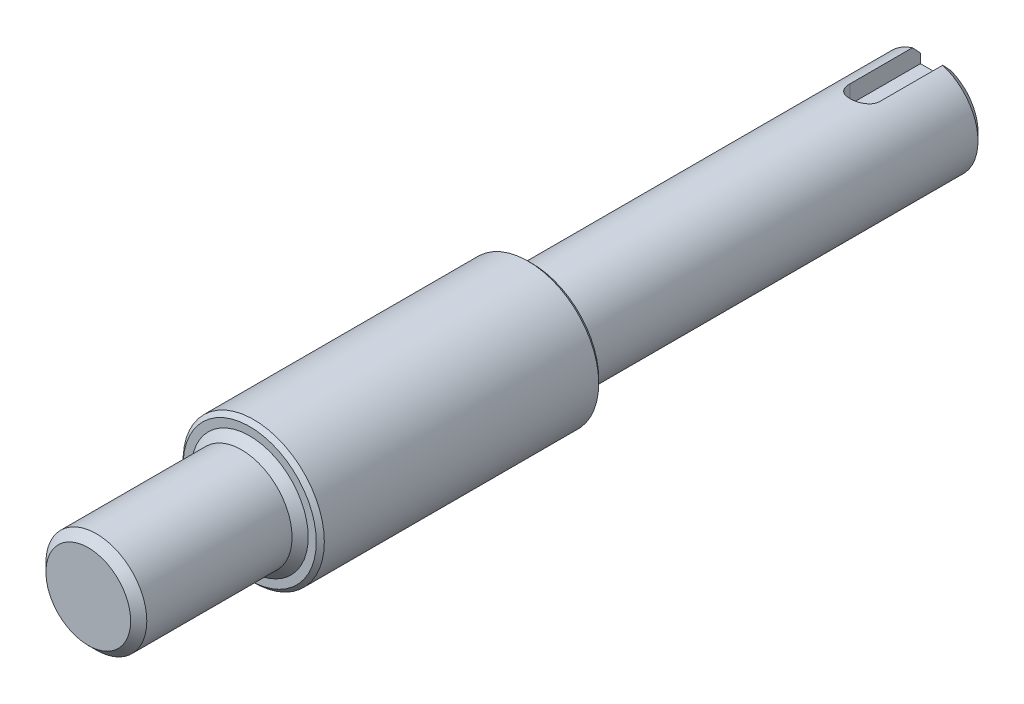
from build123d import *

# Parameters (mm, degrees)
BOSS_EXTRUDE1_DEPTH      = 400
BOSS_EXTRUDE1_DEPTH_BACK = 20
SKETCH1_R                = 25
CHAMFER1_SIZE            = 4
CUT_EXTRUDE1_DEPTH       = 10
SKETCH3_R                = 35
BOSS_EXTRUDE2_DEPTH      = 70
CHAMFER2_SIZE            = 2
CHAMFER3_SIZE            = 4


with BuildPart() as part:
    # Sketch1 → Boss-Extrude1 (new, two sides: drawn at the far end of the back side and taken through both)
    with BuildSketch(Plane.XY.offset(-BOSS_EXTRUDE1_DEPTH_BACK)):
        Circle(SKETCH1_R)
    extrude(amount=BOSS_EXTRUDE1_DEPTH + BOSS_EXTRUDE1_DEPTH_BACK)

    # Chamfer1
    chamfer1_edges = [part.edges().sort_by_distance(p)[0] for p in [
        (-25, 0, -20),
        (-25, 0, 400),
    ]]
    chamfer(chamfer1_edges, length=CHAMFER1_SIZE)

    # Sketch2 → Cut-Extrude1 (cut)
    with BuildSketch(Plane(origin=(0, 25, 0), x_dir=(1, 0, 0), z_dir=(0, 1, 0))):
        with BuildLine():
            Line((7.5, -15), (7.5, 55))
            Line((7.5, 55), (-7.5, 55))
            Line((-7.5, 55), (-7.5, -15))
            ThreePointArc((-7.5, -15), (0, -22.5), (7.5, -15))
        make_face()
    extrude(amount=-CUT_EXTRUDE1_DEPTH, mode=Mode.SUBTRACT)

    # Sketch3 → Boss-Extrude2 (add, symmetric)
    with BuildSketch(Plane.XY.offset(250)):
        Circle(SKETCH3_R)
    extrude(amount=BOSS_EXTRUDE2_DEPTH, both=True)

    # Chamfer2
    chamfer2_edges = [part.edges().sort_by_distance(p)[0] for p in [
        (-35, 0, 180),
        (-35, 0, 320),
    ]]
    chamfer(chamfer2_edges, length=CHAMFER2_SIZE)

    # Chamfer3
    chamfer3_edges = [part.edges().sort_by_distance(p)[0] for p in [
        (-25, 0, 320),
        (-25, 0, 180),
    ]]
    chamfer(chamfer3_edges, length=CHAMFER3_SIZE)


solid = part.part
